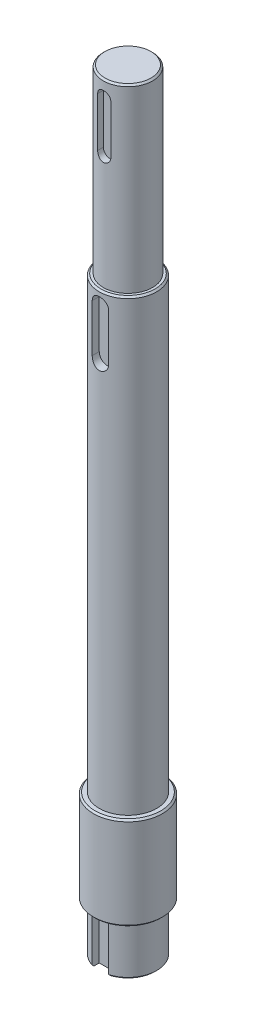
SolidWorks part; units mm, degrees
ref_plane "Front Plane" through (0, 0, 0) normal (0, 0, 1) x (1, 0, 0)
ref_plane "Top Plane" through (0, 0, 0) normal (0, 1, 0) x (1, 0, 0)
ref_plane "Right Plane" through (0, 0, 0) normal (1, 0, 0) x (0, 0, -1)
sketch "Sketch1" plane through (0, 0, 0) normal (0, 1, 0) x (1, 0, 0)
  circle A0 centre (0, 0) radius 17.5
  dimension "D1" = 35
extrude "Boss-Extrude1" add sketch "Sketch1" along normal blind 30
sketch "Sketch2" plane through (0, 30, 0) normal (0, 1, 0) x (1, 0, 0)
  circle A0 centre (0, 0) radius 21
  dimension "D1" = 42
extrude "Boss-Extrude2" add sketch "Sketch2" along normal blind 56.5
sketch "Sketch3" plane through (0, 86.5, 0) normal (0, 1, 0) x (1, 0, 0)
  circle A0 centre (0, 0) radius 17.5
  dimension "D1" = 35
extrude "Boss-Extrude3" add sketch "Sketch3" along normal blind 273.5
sketch "Sketch4" plane through (0, 360, 0) normal (0, 1, 0) x (1, 0, 0)
  circle A0 centre (0, 0) radius 15
  dimension "D1" = 30
extrude "Boss-Extrude4" add sketch "Sketch4" along normal blind 110
chamfer "Chamfer1" distance 1 angle 45 1 edges at (0, 0, 17.5)
chamfer "Chamfer3" distance 1 angle 45 4 edges at (0, 30, 21) (0, 86.5, 21) (0, 360, 17.5) (0, 470, 15)
sketch "Sketch5" plane through (0, 0, 0) normal (0, -1, 0) x (1, 0, 0)
  line L0 (0, 0) -> (0, 9.235) construction
  line L1 (-5, 22.5) -> (5, 22.5)
  line L2 (-5, 22.5) -> (-5, 12.5)
  line L3 (-5, 12.5) -> (5, 12.5)
  line L4 (5, 22.5) -> (5, 12.5)
  dimension "D1" = 12.5
  dimension "D2" = 10
  dimension "D3" = 10
extrude "Cut-Extrude1" cut sketch "Sketch5" against normal blind 30
ref_plane "Plane1" through (0, 0, 18) normal (0, 0, 1) x (1, 0, 0)
sketch "Sketch8" plane through (0, 0, 18) normal (0, 0, 1) x (1, 0, 0)
  line L0 (0, 351.5) -> (0, 322.5) construction
  line L1 (5, 351.5) -> (5, 322.5)
  line L2 (-5, 351.5) -> (-5, 322.5)
  line L4 (16.5, 360) -> (-16.5, 360) construction
  arc A0 (5, 351.5) -> (-5, 351.5) centre (0, 351.5) ccw
  arc A1 (-5, 322.5) -> (5, 322.5) centre (0, 322.5) ccw
  point P3 (0, 337)
  dimension "D1" = 29
  dimension "D2" = 10
  dimension "D3" = 23
extrude "Cut-Extrude10" cut sketch "Sketch8" against normal blind 5.5
sketch "Sketch9" plane through (0, 0, 18) normal (0, 0, 1) x (1, 0, 0)
  line L0 (0, 460) -> (0, 430) construction
  line L1 (4, 460) -> (4, 430)
  line L2 (-4, 460) -> (-4, 430)
  line L3 (14, 470) -> (-14, 470) construction
  arc A0 (4, 460) -> (-4, 460) centre (0, 460) ccw
  arc A1 (-4, 430) -> (4, 430) centre (0, 430) ccw
  point P3 (0, 445)
  dimension "D1" = 8
  dimension "D2" = 10
  dimension "D3" = 30
extrude "Cut-Extrude11" cut sketch "Sketch9" against normal blind 7
